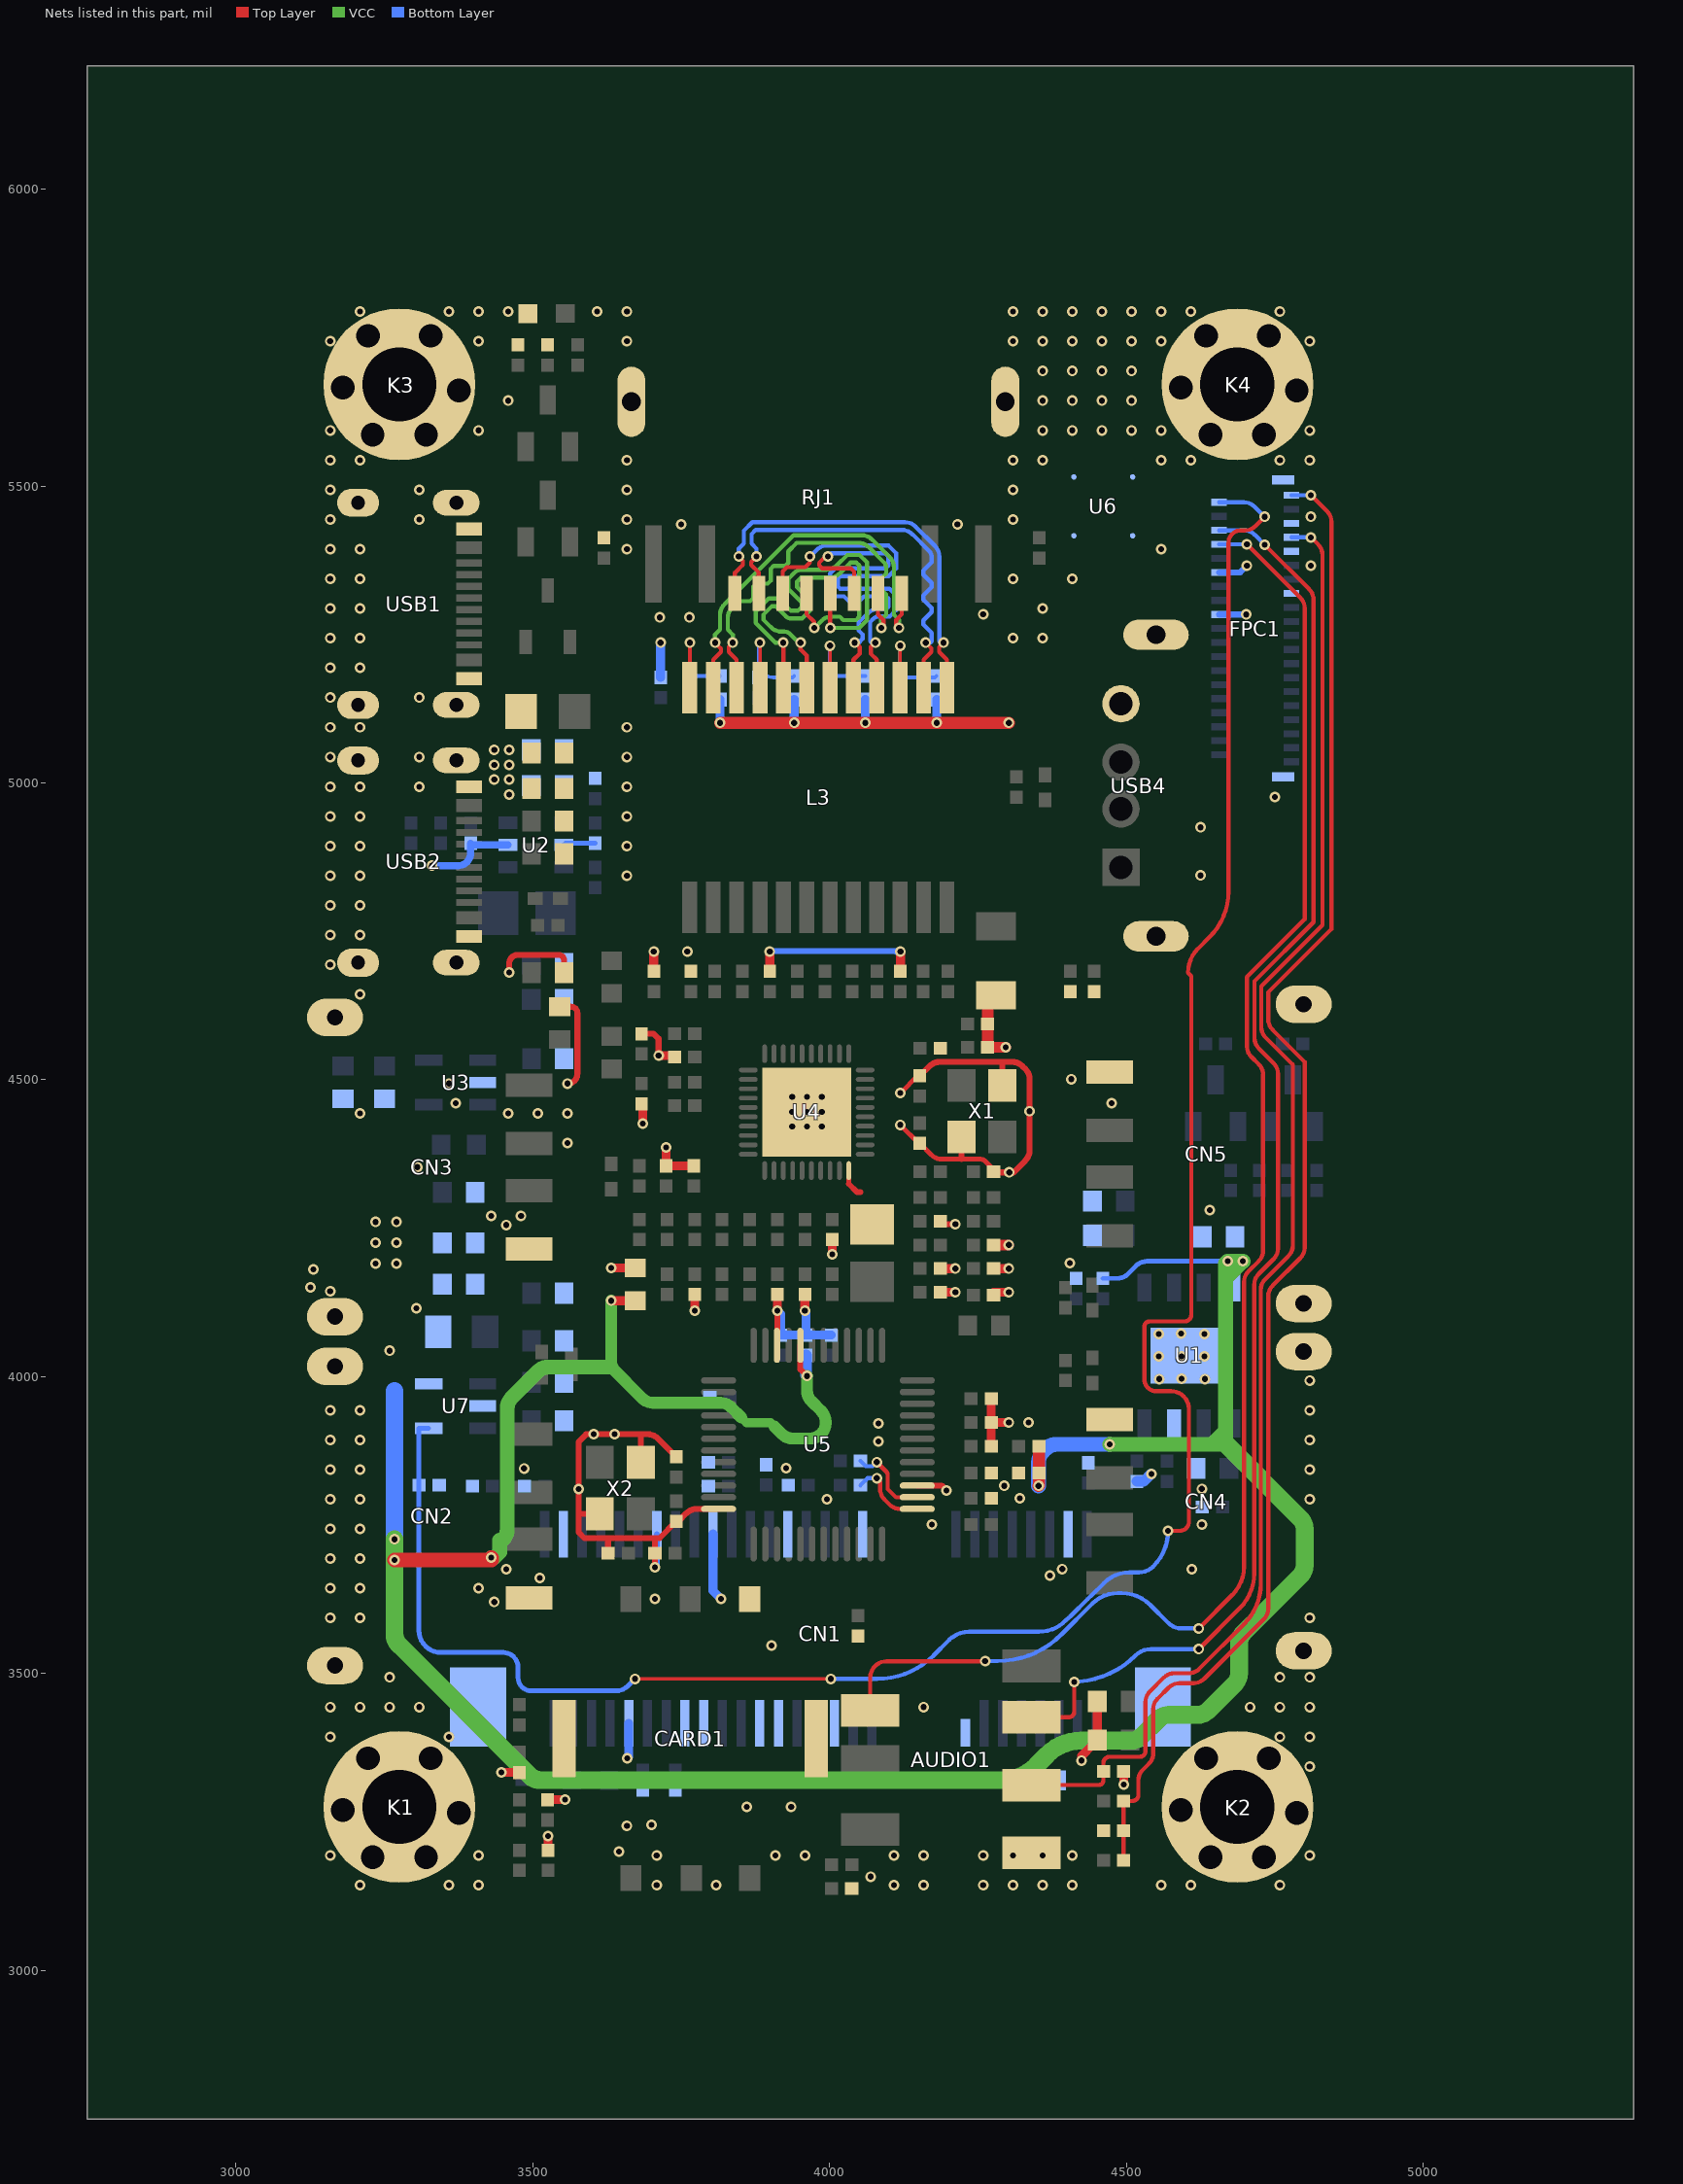
[diagram p0: the nets of this part, all layers, seen from the top]
# Altium PCB MISC84334.PcbDoc (part 6 of 8)
Units mil, origin at the board's own origin, x right, y up, seen from the top; angles counter-clockwise.
Board outline 2605.13 x 3457.4 mil, 4 copper layers (Top Layer, GND, VCC, Bottom Layer), stack 62.447 mil thick; 209 components, 149 nets, 735 pads, 529 vias.

## Via types
v1: diameter 18, hole 10, Top Layer to Bottom Layer, 529 vias

## Nets (pads, with @x,y where several pads share a name; then routed paths per layer and width w, separated by ;. In a path a pad name is that pad's centre, name@x,y a point inside that pad or via, vN(x,y) a via of type N, cw(c..) or ccw(c..) an arc to the next point about the centre after c; other vN are vias at no path point) (continued)
GND: AUDIO1.1 C1.1 C2.1 C3.1 C4.1 C5.1 C7.1 C8.1 C10.1 C11.1 C12.1 C13.1 C14.1 C15.1 C16.1 C17.1 C18.1 C19.1 C20.1 C21.1 C22.1 C23.1 C24.1 C25.1 C26.1 C27.1 C28.1 C29.1 C30.1 C31.1 C32.1 C33.1 C34.1 C35.1 C36.1 C37.1 C38.1 C39.1 C40.1 C41.1 C42.1 C43.1 C44.1 C45.1 C46.1 C47.1 C48.1 C49.1 C50.1 C51.2 C52.1 C53.1 C54.1 C55.1 C56.1 C59.2 C60.1 C61.1 C62.1 C63.1 C64.1 C65.1 C66.1 C67.1 C68.1 C69.1 C70.1 C71.1 C72.2 C73.1 C74.1 C75.1 CARD1.1 CARD1.2 CARD1.C5 CN1.4 CN1.15 CN1.18 CN1.21 CN1.26 CN1.27 CN1.29 CN1.34 CN1.35 CN1.37 CN1.40 CN1.43 CN1.50 CN1.53 CN2.4 CN2.SH1 CN2.SH2 CN3.4 CN3.SH1 CN3.SH2 CN4.4 CN4.SH1 CN4.SH2 CN5.4 CN5.SH1 CN5.SH2 CX1.1 CX2.1 D1.2 D2.2 D3.2 D4.2 D5.2 D6.2 D7.2 D8.2 FPC1.22 FPC1.25 FPC1.28 FPC1.31 FPC1.35 FPC1.40 FPC1.41 K1.1 K2.1 K3.1 K4.1 L7.1 LED1.1 R3.1 R4.1 R5.1 R6.1 R9.1 R11.1 R15.2 R17.2 R22.1 R23.2 R26.1 R30.1 R47.1 R58.2 R61.1 R73.2 R77.1 R78.1 RJ1.13 RJ1.14 U1.3 U1.9 U2.2 U3.2 U4.41 U5.10 U5.24 U5.39 U6.1 U7.2 USB1.1 USB1.12 USB1.13 USB1.14 USB2.1 USB2.12 USB2.13 USB2.14 USB4.4 USB4.5 USB4.6 X1.2 X1.4 X2.2 X2.4 | length 4556.1
  Top Layer w7: U5.10@3911.69,4052.91 U5.10@3912.23,4053.45
  Top Layer w8: v1(4119.29,4424.19) 4150.43,4393.05 CX2.1@4152.35,4393.05 4171.73,4373.67 ccw(c4189.41,4391.35) 4189.41,4366.35 4222.39,4366.35 4254.66,4366.35 cw(c4254.66,4354.99) 4262.69,4363.02 4276.63,4349.08 R23.2@4276.63,4345.09 ; v1(4119.29,4478.19) 4120.32,4478.19 4148.76,4506.63 CX1.1@4152.05,4506.63
  Top Layer w10: v1(3460.59,4680.59) 3460.59,4695.59 cw(c3475.59,4695.59) 3475.59,4710.59 3543.32,4710.59 cw(c3543.32,4700.76) 3553.15,4700.76 C69.1@3553.15,4680.59 ; C68.1@3545.59,4623.15 3564.8,4623.15 cw(c3564.8,4612.36) 3575.59,4612.36 3575.59,4510.35 cw(c3559,4510.35) v1(3559,4493.76) ; X2.4@3613.28,3769.14 3577.44,3769.14 3577.29,3769.28 ; C39.1@3627.15,3703.09 3627.15,3727.87 3627.47,3728.18 ; X2.2@3682.18,3855.76 3682.18,3902.88 3681.88,3903.19 ; C23.1@3685.59,4577.63 3703.9,4577.63 3712.29,4569.24 v1(3712.29,4541.09) ; v1(3706.1,3679.19) C45.1@3706.1,3703.09 3706.1,3727.76 3706.52,3728.18 ; C51.2@3742.02,3865.13 3711.28,3895.87 ccw(c3693.6,3878.19) 3693.6,3903.19 3681.88,3903.19 ; U5.24@3813.27,3777.32 3776.78,3777.32 ccw(c3776.78,3752.32) 3759.1,3770 3745.45,3756.35 C50.1@3742.02,3756.35 3713.85,3728.18 3706.52,3728.18 ; U5.10@3912.23,4053.45 v1(3912.23,4111.19) ; U5.39@4147.91,3816.69 4189.29,3816.69 v1(4197.29,3808.69) ; CX1.1@4152.05,4506.63 4168.28,4522.87 cw(c4185.96,4505.19) 4185.96,4530.19 4291.26,4530.19 ; R17.2@4186.69,4262.09 4191.69,4257.09 v1(4212.29,4257.09) ; 4222.39,4366.35 4222.64,4366.6 X1.2@4222.64,4403.78 ; R23.2@4276.63,4345.09 4277.63,4344.09 v1(4303.14,4344.09) 4310.14,4344.09 4329.97,4363.92 ccw(c4312.29,4381.6) 4337.29,4381.6 v1(4337.29,4447.19) 4337.29,4500.84 ccw(c4312.29,4500.84) 4329.97,4518.51 4325.61,4522.87 ccw(c4307.94,4505.19) 4307.94,4530.19 4291.26,4530.19 ; X1.4@4291.54,4490.4 4291.54,4529.91 4291.26,4530.19 ; 3577.29,3769.28 v1(3577.29,3810.69) 3577.29,3890.19 3590.29,3903.19 v1(3603.29,3903.19) v1(3638.29,3903.19) 3681.88,3903.19 ; 3577.29,3769.28 3577.29,3738.18 3587.29,3728.18 3627.47,3728.18 ; 3627.47,3728.18 3706.52,3728.18
  Top Layer w15: v1(3447.29,3333.55) D8.2@3478.04,3333.55 ; D6.2@3525.59,3287.63 v1(3554.79,3287.63) ; D5.2@3525.8,3202.63 v1(3525.8,3226.19) ; v1(3632.29,4183.15) C48.1@3673,4183.15 ; v1(3685.59,4426.19) C16.1@3685.59,4459.67 ; C32.1@3704.09,4682.63 v1(3704.09,4716.19) ; v1(3712.29,4541.09) 3736.05,4541.09 C22.1@3739.05,4538.09 ; v1(3725.09,4386.19) C24.1@3725.09,4355.13 C25.1@3771.52,4355.13 ; v1(3772.95,4111.19) R22.1@3772.95,4138.55 ; C27.1@3899.65,4682.63 v1(3899.65,4716.19) ; v1(3912.23,4111.19) R30.1@3912.23,4138.55 ; v1@3957.29,4111.19 v1(3958.66,4111.19) R26.1@3958.66,4138.55 ; v1(4005.09,4206.19) C17.1@4005.09,4230.81 ; C26.1@4119.79,4682.63 v1(4119.79,4716.19) ; C18.1@4186.63,4182.09 v1(4212.29,4182.09) ; C19.1@4186.87,4142.09 v1(4212.29,4142.09) ; C38.1@4272.64,3883.09 C37.1@4272.64,3923.09 ; C42.1@4272.64,3963.09 C37.1@4272.64,3923.09 ; C31.1@4276.63,4142.09 v1(4302.29,4142.09) ; C30.1@4276.63,4182.09 v1(4302.29,4182.09) ; v1(4302.29,3923.09) C37.1@4272.64,3923.09 ; v1(4424.79,3353.69) 4424.79,3361.48 4444.08,3380.77 ccw(c4426.4,3398.45) 4451.4,3398.45 C65.1@4451.4,3453.09 ; v1(4495.69,3313.09) R73.2@4495.69,3335.59
  Top Layer w18: C28.1@4266.52,4555.09 v1(4297.29,4555.09) ; C29.1@4276.63,4222.09 v1(4302.29,4222.09)
  Top Layer w20: v1(3815.59,5101.19) v1(3940.59,5101.19) v1(4060.59,5101.19) v1(4180.59,5101.19) v1(4302.29,5101.19) ; C28.1@4266.52,4555.09 C34.1@4266.52,4594.09 4266.52,4625.47 cw(c4273.35,4625.47) 4268.52,4630.3 C20.1@4280.59,4642.37
  Bottom Layer w10: v1(3706.1,3679.19) 3709.37,3682.45 CN1.40@3709.37,3735.04 ; v1(3899.65,4716.19) 3900.06,4716.6 4111.88,4716.6 v1@4116.29,4712.19 ; FPC1.22@4656.27,5283.71 v1(4702.29,5283.71) ; FPC1.28@4656.27,5354.57 4692.27,5354.57 v1(4703.29,5365.59)
  Bottom Layer w12: v1(3330.59,4860.59) 3374.47,4860.59 ccw(c3374.47,4881.71) 3395.59,4881.71 R11.1@3395.59,4898.55 ccw(c3398.55,4898.55) 3398.55,4895.59 U2.2@3458.35,4895.59
  Bottom Layer w15: v1(3659.29,3357.19) 3662.12,3360.02 CN1.43@3662.12,3416.14 ; C21.1@3715.59,5177.63 v1(3715.59,5236.19) ; CN1.34@3803.86,3735.04 3803.86,3639.62 v1(3817.29,3626.19) ; v1(3815.59,5101.19) D1.2@3815.59,5140.75 ; v1(3912.23,4111.19) 3918.09,4105.33 C36.1@3918.09,4070.13 C49.1@3960.59,4070.13 ; v1(3940.59,5101.19) D2.2@3940.59,5140.75 ; v1(3958.66,4111.19) 3960.59,4109.26 C49.1@3960.59,4070.13 ; C47.1@4003.09,4070.13 C49.1@3960.59,4070.13 ; v1(4060.59,5101.19) D3.2@4060.59,5140.75 ; v1(4180.59,5101.19) D4.2@4180.59,5140.75
  Bottom Layer w18: R4.1@4517.59,3823.55 4529.65,3823.55 v1@4542.05,3835.95
  other v1: 3209,3143.76 3359,3143.76 3409,3143.76 3709,3143.76 3809,3143.76 4109,3143.76 4159,3143.76 4259,3143.76 4309,3143.76 4359,3143.76 4409,3143.76 4559,3143.76 4609,3143.76 4759,3143.76 4069.79,3158.09 3159,3193.76 3409,3193.76 3709,3193.76 3909,3193.76 3959,3193.76 4109,3193.76 4159,3193.76 4259,3193.76 4309,3193.76 4359,3193.76 4409,3193.76 4809,3193.76 3645.59,3200.59 3659,3243.76 3700.59,3245.59 3860.59,3275.59 3935.59,3275.59 4809,3343.76 3159,3393.76 3359,3393.76 4759,3393.76 4809,3393.76 3159,3443.76 3209,3443.76 3259,3443.76 3309,3443.76 4159,3443.76 4709,3443.76 4759,3443.76 4809,3443.76 3259,3493.76 4759,3493.76 4809,3493.76 3902.29,3547.19 3159,3593.76 3209,3593.76 4809,3593.76 3435.59,3620.59 3706.1,3626.19 3159,3643.76 3209,3643.76 3409,3643.76 3512.35,3661.1 4371.29,3665.19 3455.59,3675.59 4392.29,3676.19 4610.59,3675.59 3159,3693.76 3209,3693.76 3159,3743.76 3209,3743.76 4172.29,3751.19 4627.29,3751.19 3995.59,3793.44 3159,3793.76 3209,3793.76 4809,3793.76 4320.59,3795.59 4627.29,3811.19 4294.79,3816.19 4542.29,3836.19 3159,3843.76 3209,3843.76 4809,3843.76 3485.59,3845.59 3927.29,3846.19 4082.29,3891.19 3159,3893.76 3209,3893.76 4809,3893.76 4082.29,3921.19 4335.59,3923.09 3159,3943.76 3209,3943.76 4809,3943.76 4809,3993.76 4555.37,3996.19 4632.29,3996.19 4593.35,3996.57 4554.98,4034.18 4631.91,4034.18 4592.97,4034.56 3259,4043.76 4554.6,4072.17 4631.53,4072.17 4592.59,4072.55 3304.11,4115.52 3159,4143.76 3125.59,4150.59 3131.05,4180.75 4405.29,4191.19 3455.59,4255.59 3430.59,4270.59 3480.59,4270.59 4640.59,4280.59 3305.59,4352.98 3559,4393.76 3937.29,4421.19 3962.29,4421.19 3987.29,4421.19 3209,4443.76 3459,4443.76 3509,4443.76 3559,4443.76 3937.29,4446.19 3962.29,4446.19 3987.29,4446.19 3370.59,4460.59 4475.59,4460.59 3937.29,4471.19 3962.29,4471.19 3987.29,4471.19 3359,4493.76 4407.29,4501.19 3209,4643.76 3159,4693.76 3760.55,4716.19 3159,4743.76 3209,4743.76 3159,4793.76 3209,4793.76 3159,4843.76 3209,4843.76 3659,4843.76 4625.29,4844.2 3159,4893.76 3209,4893.76 3659,4893.76 4625.29,4925.19 3159,4943.76 3209,4943.76 3659,4943.76 4750.29,4976.19 3159,4993.76 3209,4993.76 3309,4993.76 3659,4993.76 3159,5043.76 3309,5043.76 3659,5043.76 3159,5093.76 3209,5093.76 3659,5093.76 3159,5143.76 3309,5143.76 3159,5193.76 3209,5193.76 3159,5243.76 3209,5243.76 4309,5243.76 4359,5243.76 3714,5278.76 3764,5278.76 4259,5283.76 3159,5293.76 3209,5293.76 4359,5293.76 3159,5343.76 3209,5343.76 4309,5343.76 4409,5343.76 4811.29,5365.59 3159,5393.76 3209,5393.76 3659,5393.76 4559,5393.76 3750.59,5435.59 4215.59,5435.59 3159,5443.76 3309,5443.76 3659,5443.76 4309,5443.76 4811.29,5448.19 3159,5493.76 3309,5493.76 3659,5493.76 4309,5493.76 3159,5543.76 3209,5543.76 3659,5543.76 4309,5543.76 4359,5543.76 4559,5543.76 4609,5543.76 4759,5543.76 4809,5543.76 3159,5593.76 3409,5593.76 4359,5593.76 4409,5593.76 4459,5593.76 4509,5593.76 4559,5593.76 4809,5593.76 3459,5643.76 4359,5643.76 4409,5643.76 4459,5643.76 4509,5643.76 4359,5693.76 4409,5693.76 4459,5693.76 4509,5693.76 3159,5743.76 3409,5743.76 3659,5743.76 4309,5743.76 4359,5743.76 4409,5743.76 4459,5743.76 4509,5743.76 4559,5743.76 4809,5743.76 3209,5793.76 3359,5793.76 3409,5793.76 3459,5793.76 3609,5793.76 3659,5793.76 4309,5793.76 4359,5793.76 4409,5793.76 4459,5793.76 4509,5793.76 4559,5793.76 4609,5793.76 4759,5793.76
GPIO0_A5: FPC1.38 R77.2 U7.4 | length 3804.3
  Top Layer w6: v1(3672.29,3491.19) v1(4002.29,3491.19)
  Top Layer w7: v1(4570.59,3740.59) 4590.39,3740.59 ccw(c4590.39,3755.79) 4605.59,3755.79 4605.59,3945.54 ccw(c4575.54,3945.54) 4575.54,3975.59 4565.72,3975.59 4550.59,3975.59 cw(c4550.59,3995.59) 4530.59,3995.59 4530.59,4084.64 cw(c4539.04,4084.64) 4539.04,4093.09 4598.09,4093.09 ccw(c4598.09,4104.59) 4609.59,4104.59 4609.59,4674.85 4604.09,4680.35 cw(c4661.41,4680.35) 4620.88,4720.88 4640.46,4740.45 ccw(c4563.6,4817.31) 4672.29,4817.31 4672.29,5404.71 cw(c4692.78,5404.71) 4678.29,5419.19 4678.76,5419.66 cw(c4692.11,5406.31) 4692.11,5425.19 4699.94,5425.19 ccw(c4699.94,5450.19) 4717.61,5432.51 v1(4733.29,5448.19)
  Bottom Layer w7: v1(4002.29,3491.19) 4080.47,3491.19 ccw(c4080.47,3625.71) 4175.59,3530.59 4201.45,3556.45 cw(c4235.59,3522.31) 4235.59,3570.59 4352.81,3570.59 ccw(c4352.81,3634.52) 4382.18,3577.74 ccw(c4352.81,3634.52) 4398.02,3589.32 ccw(c4305.59,3699.1) 4407.07,3597.62 4435.13,3625.69 cw(c4485.59,3575.24) 4440.7,3630.7 4462.91,3652.91 cw(c4505.59,3610.24) 4505.59,3670.59 4521.45,3670.59 ccw(c4521.45,3704.73) 4545.59,3680.59 4545.84,3680.84 ccw(c4486.09,3740.59) v1(4570.59,3740.59) ; FPC1.38@4656.27,5472.68 4698.45,5472.68 cw(c4698.45,5447.68) 4716.12,5465.36 v1(4733.29,5448.19)
  Bottom Layer w8: U7.4@3325.17,3913.19 3308.55,3913.19 R77.2@3308.55,3817.49 3308.55,3572.63 ccw(c3345.59,3572.63) 3345.59,3535.59 3450.59,3535.59 cw(c3450.59,3510.59) 3475.59,3510.59 3475.59,3492.89 ccw(c3497.29,3492.89) 3497.29,3471.19 3641.94,3471.19 ccw(c3641.94,3496.19) 3659.61,3478.51 v1(3672.29,3491.19)
GPIO0_C5: C59.1 FPC1.39 R74.1 R75.1 | length 2567.8
  Top Layer w7: R74.1@4495.69,3185.59 C59.1@4495.69,3235.59 R75.1@4495.69,3285.59 4510.59,3285.59 ccw(c4510.59,3295.43) 4520.43,3295.43 4520.43,3320.24 cw(c4545.43,3320.24) 4527.75,3337.91 4538.27,3348.43 ccw(c4520.59,3366.11) 4545.59,3366.11 4545.59,3440.24 cw(c4570.59,3440.24) 4552.91,3457.91 4571.59,3476.59 cw(c4589.27,3458.92) 4589.27,3483.92 4613.56,3483.92 ccw(c4613.56,3508.92) 4631.24,3491.24 4731.88,3591.88 ccw(c4714.2,3609.56) 4739.2,3609.56 4739.2,4135.57 cw(c4764.2,4135.57) 4746.53,4153.25 4793.27,4199.99 ccw(c4775.59,4217.67) 4800.59,4217.67 4800.59,4530.4 4746.53,4584.46 cw(c4764.2,4602.14) 4739.2,4602.14 4739.2,4647.17 4845.59,4753.55 4845.59,5439.85 ccw(c4820.59,5439.85) 4838.27,5457.52 v1(4811.29,5484.5)
  Bottom Layer w7: FPC1.39@4778.31,5484.5 v1(4811.29,5484.5)
HP_SNS: AUDIO1.2 FPC1.33 R73.1 | length 2504.4
  Top Layer w7: AUDIO1.2@4340.45,3312.29 4453.31,3312.29 ccw(c4453.31,3320.59) 4461.61,3320.59 R73.1@4461.61,3335.59 4461.61,3349.67 cw(c4471.92,3349.67) 4471.92,3359.97 4523.14,3359.97 ccw(c4523.14,3369.3) 4532.47,3369.3 4532.47,3452.11 cw(c4557.47,3452.11) 4539.79,3469.79 4563.27,3493.27 cw(c4580.95,3475.59) 4580.95,3500.59 4605.24,3500.59 ccw(c4605.24,3525.59) 4622.91,3507.91 4698.66,3583.66 ccw(c4631.24,3651.09) 4726.59,3651.09 4726.59,4146.24 cw(c4751.59,4146.24) 4733.91,4163.91 4773.27,4203.27 ccw(c4755.59,4220.95) 4780.59,4220.95 4780.59,4525.59 4734.97,4571.21 cw(c4752.64,4588.89) 4727.64,4588.89 4727.64,4657.64 4830.59,4760.59 4830.59,5383.98 ccw(c4805.59,5383.98) 4823.27,5401.65 v1(4811.29,5413.63)
  Bottom Layer w7: FPC1.33@4778.31,5413.63 v1(4811.29,5413.63)
HPL_OUT: AUDIO1.4 FPC1.32 | length 2684.6
  Top Layer w7: AUDIO1.4@4068.8,3438.27 4068.8,3493.27 cw(c4096.35,3493.27) 4096.35,3520.82 v1@4262.93,3520.82 ; v1(4622.29,3576.19) 4678.85,3632.75 ccw(c4631.44,3680.16) 4698.49,3680.16 4698.49,4159.75 cw(c4723.49,4159.75) 4705.81,4177.43 4723.27,4194.89 ccw(c4705.59,4212.57) 4730.59,4212.57 4730.59,4508.5 ccw(c4705.59,4508.5) 4723.27,4526.17 4710.62,4538.82 cw(c4728.3,4556.49) 4703.3,4556.49 4703.3,4673.3 4800.59,4770.59 4800.59,5294.17 ccw(c4775.59,5294.17) 4793.27,5311.84 v1(4703.29,5401.82)
  Bottom Layer w7: v1(4262.29,3521.19) 4283.31,3521.19 ccw(c4283.31,3673.01) 4390.66,3565.66 4442.91,3617.91 cw(c4485.59,3575.24) 4485.59,3635.59 4492.31,3635.59 cw(c4492.31,3567.31) 4540.59,3615.59 4571.07,3585.11 ccw(c4592.61,3606.64) 4592.61,3576.19 v1(4622.29,3576.19) ; FPC1.32@4656.27,5401.82 v1(4703.29,5401.82)
HPR_OUT: AUDIO1.3 FPC1.34 | length 2444
  Top Layer w7: AUDIO1.3@4340.45,3426.46 4403.16,3426.46 ccw(c4403.16,3435.59) 4412.29,3435.59 v1(4412.29,3486.19) ; v1(4622.29,3541.19) 4691.2,3610.1 ccw(c4632.31,3668.99) 4715.59,3668.99 4715.59,4155.24 cw(c4740.59,4155.24) 4722.91,4172.91 4748.27,4198.27 ccw(c4730.59,4215.95) 4755.59,4215.95 4755.59,4510.24 ccw(c4730.59,4510.24) 4748.27,4527.91 4723.46,4552.72 cw(c4741.14,4570.39) 4716.14,4570.39 4716.14,4666.14 4815.59,4765.59 4815.59,5308.54 ccw(c4790.59,5308.54) 4808.27,5326.21 v1(4733.29,5401.19)
  Bottom Layer w7: v1(4412.29,3486.19) 4408.4,3486.19 ccw(c4408.4,3637.78) 4515.59,3530.59 cw(c4541.18,3505) 4541.18,3541.19 v1(4622.29,3541.19) ; FPC1.34@4656.27,5425.44 4698.69,5425.44 cw(c4698.69,5400.44) 4716.36,5418.12 v1(4733.29,5401.19)
HUB_DM7: R68.2 U5.37 | length 133.3
  Top Layer w7: v1(4079.79,3829.19) 4085.29,3823.69 4085.29,3811.15 ccw(c4110.29,3811.15) 4092.61,3793.47 4101.44,3784.64 ccw(c4119.12,3802.32) 4119.12,3777.32 U5.37@4147.91,3777.32
  Bottom Layer w7: R68.2@4052.33,3817.19 4064.33,3829.19 v1(4079.79,3829.19)
HUB_DP7: R69.2 U5.38 | length 142
  Top Layer w7: v1(4079.79,3856.19) 4096.01,3839.97 cw(c4090.5,3834.46) 4098.29,3834.46 4098.29,3811.01 4112.29,3797.01 U5.38@4147.91,3797.01
  Bottom Layer w7: R69.2@4052.33,3858.19 4061.33,3849.19 4072.79,3849.19 v1(4079.79,3856.19)
IN_5V: C1.2 C2.2 C3.2 C7.2 C8.2 C43.2 C48.2 C49.2 C72.1 C73.2 F1.2 R2.2 R7.2 R60.2 R76.1 U1.8 U2.5 U5.8 U7.5 | length 5052.4
  Top Layer w10: U5.8@3951.06,4052.91 3951.06,4012.42 v1(3962.29,4001.19)
  Top Layer w15: v1(3632.29,4128.03) C48.2@3673,4128.03
  Top Layer w20: v1(4352.29,3816.19) 4352.99,3816.89 C43.2@4352.99,3838.09 R60.2@4352.99,3883.09
  Top Layer w25: v1(3267.29,3691.19) 3431.19,3691.19 3430.59,3691.79 v1(3430.59,3695.59)
  VCC w15: 3851.56,3931.32 3860.3,3922.59 3900.89,3922.59 3907.29,3916.19
  VCC w20: v1(3632.29,4128.03) 3632.29,4016.19 3684.97,3963.51 ccw(c3702.65,3981.19) 3702.65,3956.19 3816.34,3956.19 cw(c3816.34,3931.19) 3834.02,3948.87 3851.56,3931.32 ; 3907.29,3916.19 3919.97,3903.51 ccw(c3937.65,3921.19) 3937.65,3896.19 3968.13,3896.19 ccw(c3968.13,3921.19) 3985.81,3903.51 3986.39,3904.1 ccw(c3968.72,3921.78) 3993.72,3921.78 3993.72,3924.41 ccw(c3968.72,3924.41) 3986.39,3942.09 3969.61,3958.87 cw(c3987.29,3976.55) 3962.29,3976.55 v1(3962.29,4001.19)
  VCC w25: v1(3430.59,3695.59) 3435.59,3695.59 3444.59,3704.59 3444.59,3724.97 3449.97,3724.97 ccw(c3432.29,3742.65) 3457.29,3742.65 3457.29,3946.94 cw(c3482.29,3946.94) 3464.61,3964.61 3508.87,4008.87 cw(c3526.55,3991.19) 3526.55,4016.19 3632.29,4016.19 ; v1(4472.29,3886.19) 4644.58,3886.19 ; 4644.58,3886.19 4664.51,3906.12 ccw(c4657.78,3912.84) 4667.29,3912.84 ; 4644.58,3886.19 4666.08,3886.19 4667.29,3887.4 4667.29,3912.84 ; 4667.29,3912.84 4667.29,4165.07 ; 4667.29,4165.07 v1(4696.67,4194.45) v1(4670.77,4194.45) 4667.29,4190.97 4667.29,4165.07
  VCC w30: v1(3267.29,3726.19) v1(3267.29,3691.19) 3267.29,3566.33 ccw(c3292.29,3566.33) 3274.61,3548.65 3495.35,3327.91 ccw(c3513.03,3345.59) 3513.03,3320.59 4289.69,3320.59 ccw(c4289.69,3403.2) 4348.1,3344.79 4366.91,3363.59 cw(c4423.89,3306.61) 4423.89,3387.19 4507.94,3387.19 ccw(c4507.94,3412.19) 4525.61,3394.51 4554.37,3423.27 cw(c4572.05,3405.59) 4572.05,3430.59 4620.24,3430.59 ccw(c4620.24,3455.59) 4637.91,3437.91 4682.9,3482.9 ccw(c4665.22,3500.57) 4690.22,3500.57 4690.22,3551.19 cw(c4715.22,3551.19) 4697.54,3568.87 4793.27,3664.59 ccw(c4775.59,3682.27) 4800.59,3682.27 4800.59,3743.74 ccw(c4775.59,3743.74) 4793.27,3761.42 4667.29,3887.4
  Bottom Layer w8: U2.5@3552.84,4895.59 3555.8,4898.55 R7.2@3605.59,4898.55 ; R2.2@4460.59,4165.58 4485.1,4165.58 ccw(c4485.1,4190.58) 4502.78,4172.9 4517.01,4187.13 cw(c4534.69,4169.45) 4534.69,4194.45 v1(4670.77,4194.45)
  Bottom Layer w20: C49.2@3960.59,4036.05 3960.59,4002.89 v1(3962.29,4001.19)
  Bottom Layer w25: v1(4352.29,3816.19) 4352.29,3855.84 cw(c4377.29,3855.84) 4359.61,3873.51 4364.97,3878.87 cw(c4382.65,3861.19) 4382.65,3886.19 v1(4472.29,3886.19)
  Bottom Layer w30: v1@3267.29,3690.59 v1(3267.29,3691.19) v1(3267.29,3726.19) 3267.29,3975.59
  other v1: 3235.59,4190.59 3270.59,4190.59 3235.59,4225.59 3270.59,4225.59 3235.59,4260.59 3270.59,4260.59 3460.59,4980.59 3435.59,5005.59 3460.59,5005.59 3435.59,5030.59 3460.59,5030.59 3435.59,5055.59 3460.59,5055.59
LAN1_A+: L3.13 RJ1.1 | length 715.6
  Top Layer w7: RJ1.1@3840.89,5319.17 3840.89,5353.98 3854.24,5367.33 3854.24,5374.24 v1(3847.29,5381.19) ; v1(4192.29,5236.19) 4184.8,5228.69 4184.8,5220.62 4197.98,5207.44 L3.13@4197.98,5160.63
  Bottom Layer w7: v1(3847.29,5381.19) 3847.29,5394.69 3855.79,5403.19 3855.79,5424.69 3870.29,5439.19 4127.32,5439.19 cw(c4127.32,5414.19) 4145,5431.87 4177.97,5398.9 cw(c4160.29,5381.22) 4185.29,5381.22 4185.29,5238.67 4187.77,5236.19 v1(4192.29,5236.19)
LAN1_A-: L3.14 RJ1.2 | length 712.3
  Top Layer w7: v1(3877.29,5381.19) 3868.08,5371.98 3868.08,5367.23 3881.05,5354.25 RJ1.2@3881.05,5319.17 ; L3.14@4158.61,5160.63 4158.61,5207.44 4171.8,5220.62 4171.8,5226.69 v1(4162.29,5236.19)
  Bottom Layer w7: v1(3877.29,5381.19) 3877.29,5394.69 3868.79,5403.19 3868.79,5419.19 3875.79,5426.19 4121.94,5426.19 cw(c4121.94,5401.19) 4139.61,5418.87 4168.18,5390.3 cw(c4158.26,5380.38) 4172.29,5380.38 4172.29,5371.72 4158.29,5357.72 4158.29,5350.72 4172.29,5336.72 4172.29,5329.72 4158.29,5315.72 4158.29,5308.72 4172.29,5294.72 4172.29,5287.72 4158.29,5273.72 4158.29,5266.72 4172.29,5252.72 4172.29,5238.67 4169.82,5236.19 v1(4162.29,5236.19)
LAN1_B+: L3.16 RJ1.3 | length 706.4
  Top Layer w7: RJ1.3@3921.21,5319.17 3921.21,5356.31 3928.27,5363.37 3959.37,5363.37 3967.29,5371.29 v1(3967.29,5381.19) ; v1(4077.29,5236.19) 4076.68,5236.19 4069.67,5229.18 4069.67,5217.63 4079.86,5207.44 L3.16@4079.86,5160.63
  Bottom Layer w7: v1(3967.29,5381.19) 3978.47,5392.37 cw(c3996.15,5374.69) 3996.15,5399.69 4099.79,5399.69 4112.29,5387.19 4112.29,5360.87 4099.61,5348.19 4018.38,5348.19 4014.07,5343.88 4014.07,5331.02 4017.9,5327.19 4101.11,5327.19 4112.29,5316.01 4112.29,5291.19 4101.29,5280.19 4082.98,5280.19 ccw(c4082.98,5267.62) 4074.08,5276.51 4068.79,5271.21 4068.79,5238.67 4071.27,5236.19 v1(4077.29,5236.19)
LAN1_B-: L3.17 RJ1.6 | length 699
  Top Layer w7: v1(3997.29,5381.19) 3993.45,5381.19 3982.85,5370.59 3982.85,5366.3 3987.77,5361.38 4036.18,5361.38 4041.68,5355.88 RJ1.6@4041.68,5319.17 ; L3.17@4040.5,5160.63 4040.5,5207.44 4050.97,5217.9 4050.97,5228.9 4043.68,5236.19 v1(4042.29,5236.19)
  Bottom Layer w7: v1(3997.29,5381.19) 4002.79,5386.69 4094.41,5386.69 4099.29,5381.81 4099.29,5366.25 4094.23,5361.19 4009.29,5361.19 4001.07,5352.97 4001.07,5321.41 4008.29,5314.19 4024.31,5314.19 4038.31,5300.19 4044.31,5300.19 4058.31,5314.19 4095.73,5314.19 4099.29,5310.63 4099.29,5296.58 4095.91,5293.19 4082.74,5293.19 ccw(c4082.74,5268.19) 4065.06,5285.87 4049.29,5270.1 4049.29,5256.8 4055.79,5250.3 4055.79,5242.61 4049.37,5236.19 v1(4042.29,5236.19)
LAN1_C+: L3.19 RJ1.4 | length 677.6
  Top Layer w7: v1(3951.29,5236.19) 3951.29,5224.89 3961.76,5214.42 L3.19@3961.76,5160.63 ; RJ1.4@3961.36,5319.17 3961.36,5284.28 3974.29,5271.35 v1(3974.29,5261.19)
  VCC w7: v1(3951.29,5236.19) 3948.45,5236.19 3934,5250.64 ccw(c3923.81,5240.45) 3923.81,5254.86 3919.25,5254.86 cw(c3919.25,5279.86) 3901.58,5262.18 3888.8,5274.96 3888.8,5283.31 3903.26,5297.77 3909.28,5297.77 3926.55,5280.5 ccw(c3934.97,5288.92) 3934.96,5277.02 3954.12,5277.02 3966.85,5289.75 3966.85,5308.63 3945.43,5330.05 3945.43,5338.99 3952.43,5345.99 4000.12,5345.99 ccw(c4000.12,5370.99) 4017.8,5353.31 4035.53,5371.05 4045.43,5371.05 4050.29,5366.19 4050.29,5279.58 4044.93,5274.22 4023.26,5274.22 4017.71,5279.78 4001.58,5279.78 ccw(c4001.58,5260.79) 3988.15,5274.21 v1@3975.13,5261.19 ; v1(3974.29,5261.19) v1@3975.13,5261.19 ; v1@3975.71,5261.19 v1@3975.13,5261.19
LAN1_C-: L3.20 RJ1.5 | length 685.5
  Top Layer w7: v1(3922.29,5236.19) 3922.39,5236.09 L3.20@3922.39,5160.63 ; v1(4001.29,5261.19) 4001.29,5318.94 RJ1.5@4001.52,5319.17
  VCC w7: v1@3922.22,5236.26 3909.11,5236.26 3875.8,5269.57 3875.8,5288.7 3897.87,5310.77 3914.67,5310.77 3935.42,5290.02 3946.85,5290.02 3953.85,5297.02 3953.85,5303.24 3930.91,5326.19 3930.91,5343.81 ; 3930.91,5344.09 3930.91,5343.81 ; v1(4001.29,5261.19) 4050.32,5261.22 4063.29,5274.19 4063.29,5371.58 4050.82,5384.05 4030.15,5384.05 4012.41,5366.31 cw(c3994.74,5383.99) 3994.74,5358.99 3952.62,5358.99 ccw(c3952.62,5343.23) 3941.47,5354.37 3930.91,5343.81
LAN1_D+: L3.22 RJ1.7 | length 686.7
  Top Layer w7: v1(3837.29,5236.19) 3830.46,5229.36 3830.46,5220.63 3843.65,5207.44 L3.22@3843.65,5160.63 ; RJ1.7@4081.84,5319.17 4081.84,5283.7 4091.24,5274.3 4091.24,5265.14 v1(4087.29,5261.19)
  VCC w7: v1(3837.29,5236.19) 3837.29,5249.69 3828.79,5258.19 3828.79,5277.79 cw(c3853.79,5277.79) 3836.11,5295.47 3846.62,5305.98 3866.42,5305.98 3871.37,5310.93 3871.37,5330.72 3876.32,5335.67 3896.12,5335.67 3901.07,5340.62 3901.07,5360.42 3906.02,5365.37 3925.82,5365.37 3930.77,5370.32 3930.77,5390.12 3944.84,5404.19 4048.94,5404.19 cw(c4048.94,5379.19) 4066.61,5396.87 4091.69,5371.79 cw(c4081.79,5361.89) 4095.79,5361.89 4095.79,5352.56 4081.79,5338.56 4081.79,5331.56 4095.79,5317.56 4095.79,5283.19 4087.29,5274.69 v1(4087.29,5261.19)
LAN1_D-: L3.23 RJ1.8 | length 684.5
  Top Layer w7: L3.23@3804.27,5160.63 3804.27,5207.44 3817.46,5220.63 3817.46,5226.19 3807.46,5236.19 v1(3807.29,5236.19) ; v1(4117.29,5261.19) 4112.46,5266.03 4112.46,5274.43 4121.99,5283.97 RJ1.8@4121.99,5319.17
  VCC w7: v1(3807.29,5236.19) 3807.29,5249.69 3815.79,5258.19 3815.79,5283.17 cw(c3840.79,5283.17) 3823.11,5300.85 3937.56,5415.29 cw(c3942.14,5410.71) 3942.14,5417.19 4054.32,5417.19 cw(c4054.32,5392.19) 4072,5409.87 4101.47,5380.4 cw(c4083.79,5362.72) 4108.79,5362.72 4108.79,5283.19 4117.29,5274.69 v1(4117.29,5261.19)
LAN1_MCT1: D1.1 L3.24 R40.2 | length 185.4
  Top Layer w6: L3.24@3764.9,5160.63 v1(3764.9,5236.19)
  Bottom Layer w6: v1(3764.9,5236.19) 3765.59,5235.5 R40.2@3765.59,5177.63 3768.08,5180.12 D1.1@3815.59,5180.12
LAN1_MCT2: D2.1 L3.21 R39.2 | length 185.4
  Top Layer w6: L3.21@3883.02,5160.63 v1(3883.02,5236.19)
  Bottom Layer w6: v1(3883.02,5236.19) 3880.59,5233.76 3880.59,5202.63 ccw(c3905.59,5202.63) 3905.59,5177.63 3938.1,5177.63 D2.1@3940.59,5180.12
LAN1_MCT3: D3.1 L3.18 R38.2 | length 185.4
  Top Layer w6: L3.18@4001.13,5160.63 v1(4001.13,5231.19)
  Bottom Layer w6: v1(4001.13,5231.19) 4000.59,5230.65 R38.2@4000.59,5177.63 4003.08,5180.12 D3.1@4060.59,5180.12
LAN1_MCT4: D4.1 L3.15 R37.2 | length 185.7
  Top Layer w6: L3.15@4119.23,5160.63 v1(4119.23,5231.19)
  Bottom Layer w6: v1(4119.23,5231.19) 4119.23,5178.99 R37.2@4120.59,5177.63 4178.1,5177.63 D4.1@4180.59,5180.12
LDO_OUT: L2.1 U4.30 | length 47.6
  Top Layer w8: 4032.66,4324.82 U4.30@4032.66,4347.19
  Top Layer w10: 4032.66,4324.82 4046.29,4311.19 4052.29,4311.19